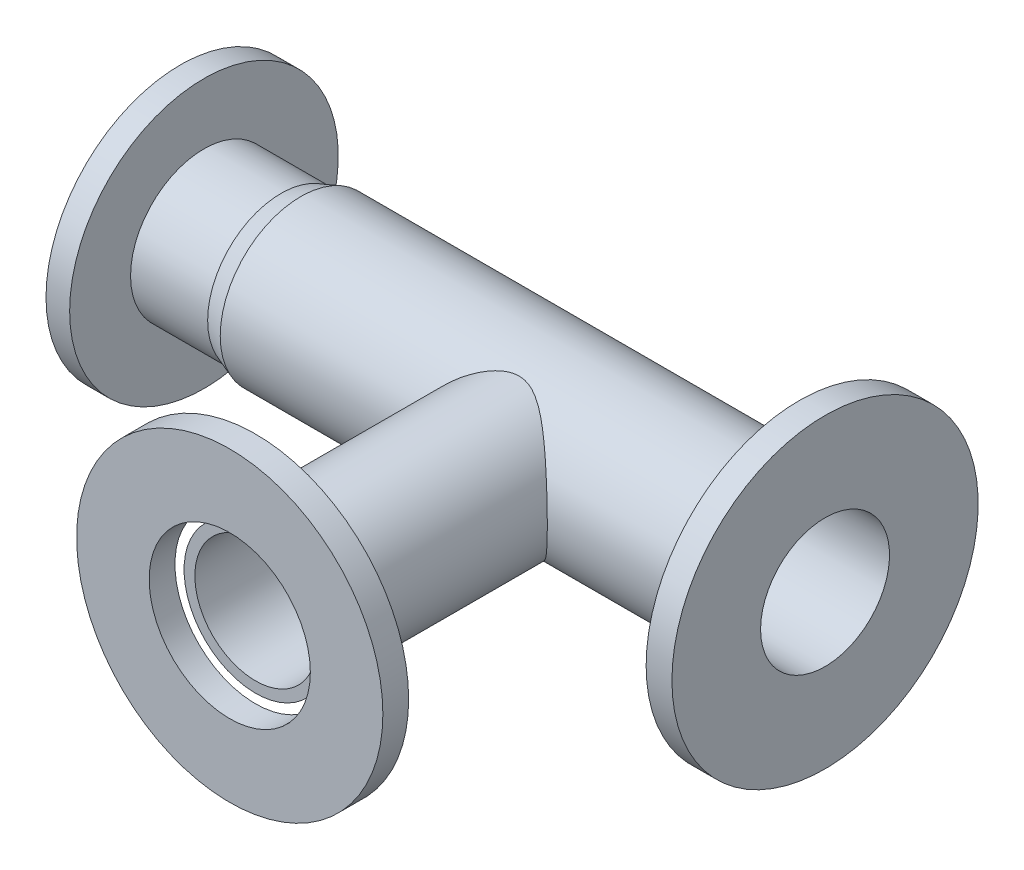
from build123d import *

# Parameters (mm, degrees)
SKETCH2_R           = 66.5
SKETCH2_R_2         = 56.5
BOSS_EXTRUDE1_DEPTH = 280
SKETCH3_R           = 142.5
SKETCH3_R_2         = 75
BOSS_EXTRUDE2_DEPTH = 24


with BuildPart() as part:
    # Sketch1 → Revolve1 (revolve)
    with BuildSketch(Plane.XY, mode=Mode.PRIVATE) as revolve1_sk:
        Polygon((0, 60), (0, 125), (22, 125), (22, 68.30000917), (93.737852553, 68.30000917), (112.145926068, 75), (576, 75), (576, 142.5), (600, 142.5), (600, 60), align=None)
    revolve(revolve1_sk.sketch.rotate(Axis((0, 0, 0), (1, 0, 0)), 90), axis=Axis((0, 0, 0), (1, 0, 0)))

    # Sketch2 → Boss-Extrude1 (add)
    with BuildSketch(Plane.XY):
        with Locations((350, 0)):
            Circle(SKETCH2_R)
        with Locations((350, 0)):
            Circle(SKETCH2_R_2, mode=Mode.SUBTRACT)
    extrude(amount=BOSS_EXTRUDE1_DEPTH)


with BuildPart() as body_2:
    # Sketch3 → Boss-Extrude2 (new body)
    with BuildSketch(Plane.XY.offset(280)):
        with Locations((350, 0)):
            Circle(SKETCH3_R)
        with Locations((350, 0)):
            Circle(SKETCH3_R_2, mode=Mode.SUBTRACT)
    extrude(amount=BOSS_EXTRUDE2_DEPTH)


solid = Compound([part.part, body_2.part])
